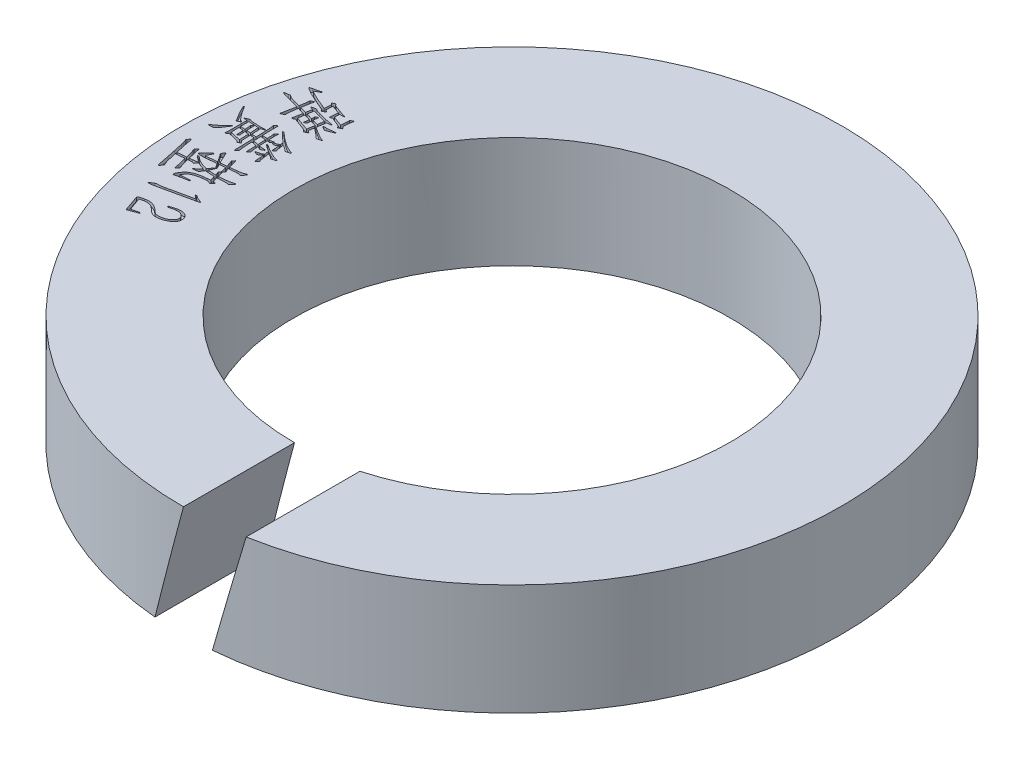
SolidWorks part; units mm, degrees
ref_plane "Front Plane" through (0, 0, 0) normal (0, 0, 1) x (1, 0, 0)
ref_plane "Top Plane" through (0, 0, 0) normal (0, 1, 0) x (1, 0, 0)
ref_plane "Right Plane" through (0, 0, 0) normal (1, 0, 0) x (0, 0, -1)
sketch "Sketch2" plane through (0, 0, 0) normal (0, 1, 0) x (1, 0, 0)
  circle A0 centre (0, 0) radius 9.2
  circle A1 centre (0, 0) radius 6.1
extrude "Boss-Extrude1" add sketch "Sketch2" along normal blind 3.1
sketch "Sketch3" plane through (0, 0, 0) normal (0, 0, 1) x (1, 0, 0)
  line L0 (-0.8023, 0) -> (0.0283, 3.1)
  line L1 (-9.2, 0) -> (9.2, 0) construction
  line L2 (9.2, 3.1) -> (-9.2, 3.1) construction
  line L3 (0.0283, 3.1) -> (1.633, 3.1)
  line L4 (6.1, 3.1) -> (-6.1, 3.1) construction
  line L5 (1.633, 3.1) -> (0.8023, 0)
  line L6 (0.8023, 0) -> (-0.8023, 0)
  line L7 (0, 0.2823) -> (0, -0.3539) construction
extrude "Cut-Extrude1" cut sketch "Sketch3" along normal through all
sketch "Sketch4" plane through (0, 3.1, 0) normal (0, 1, 0) x (1, 0, 0)
  circle A0 centre (0, 0) radius 8.5796 construction
  text T0 "弹簧垫12" font "汉仪长仿宋体" height in points 5
extrude "Cut-Extrude2" cut sketch "Sketch4" against normal blind 0.1
equation "\"d1\"= 12.2"
equation "\"s\"= 3.1"
equation "\"b\"= 3.1"
equation "\"h\"= 7.75"
equation "\"m\"= 1.55"
equation "\"D1@Sketch2\"=\"d1\""
equation "\"D2@Sketch2\"=\"b\""
equation "\"D1@Boss-Extrude1\"=\"s\""
equation "\"D1@Sketch3\"=\"m\""
